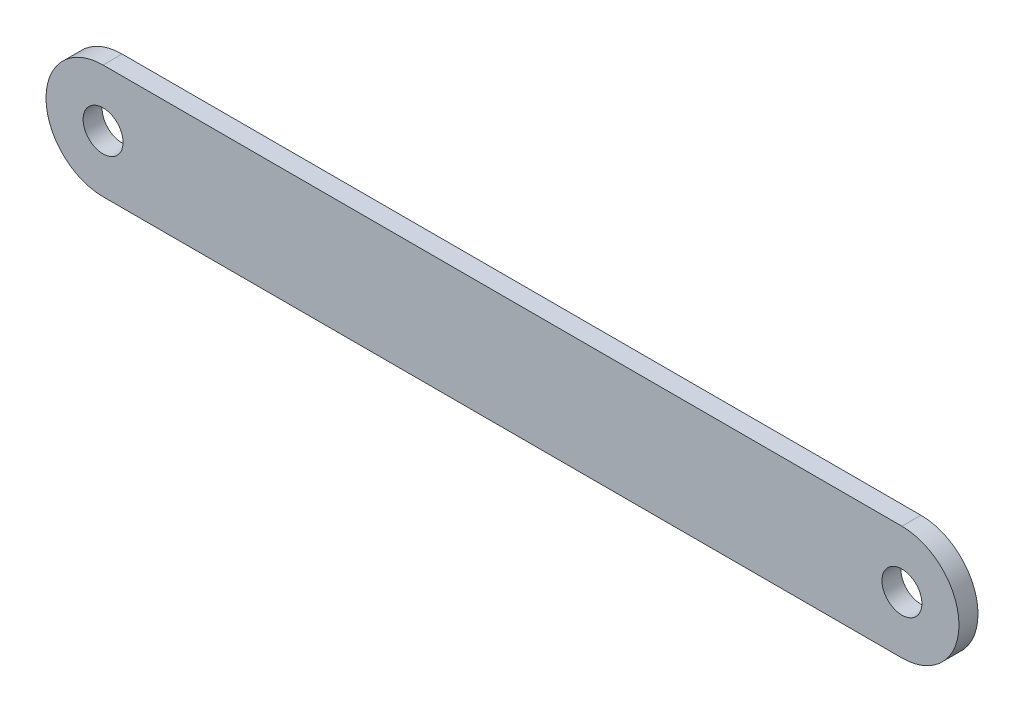
SolidWorks part; units mm, degrees
ref_plane "Front" through (0, 0, 0) normal (0, 0, 1) x (1, 0, 0)
ref_plane "Top" through (0, 0, 0) normal (0, 1, 0) x (1, 0, 0)
ref_plane "Right" through (0, 0, 0) normal (1, 0, 0) x (0, 0, -1)
sketch "Sketch1" plane through (0, 0, 0) normal (0, 0, 1) x (1, 0, 0)
  line L0 (0, 0) -> (84, 0) construction
  line L1 (0, 6) -> (84, 6)
  line L2 (0, -6) -> (84, -6)
  arc A0 (0, 6) -> (0, -6) centre (0, 0) ccw
  arc A1 (84, -6) -> (84, 6) centre (84, 0) ccw
  point P3 (42, 0)
  dimension "D1" = 84
  dimension "D2" = 12
extrude "Boss-Extrude1" add sketch "Sketch1" along normal mid plane 2
hole_wizard "Ø4.2 (4.2) Diameter Hole1" positions "Sketch3" profile "Sketch2" hole size "Ø4.2" standard "Gb" end condition through all
sketch "Sketch3" plane through (0, 0, 1) normal (0, 0, 1) x (1, 0, 0)
  point P0 (0, 0)
  point P3 (84, 0)
sketch "Sketch2" plane through (0, 0, 1) normal (1, 0, 0) x (0, -1, 0)
  line L0 (0, 0) -> (0, 2)
  line L1 (0, 2) -> (2.1, 2)
  line L2 (2.1, 2) -> (2.1, 0)
  line L5 (2.1, 0) -> (0, 0)
  line L11 (0, -6.35) -> (0, 107.95) construction
  dimension "通孔孔直径" = 4.2
  dimension "通孔孔深度" = 2
